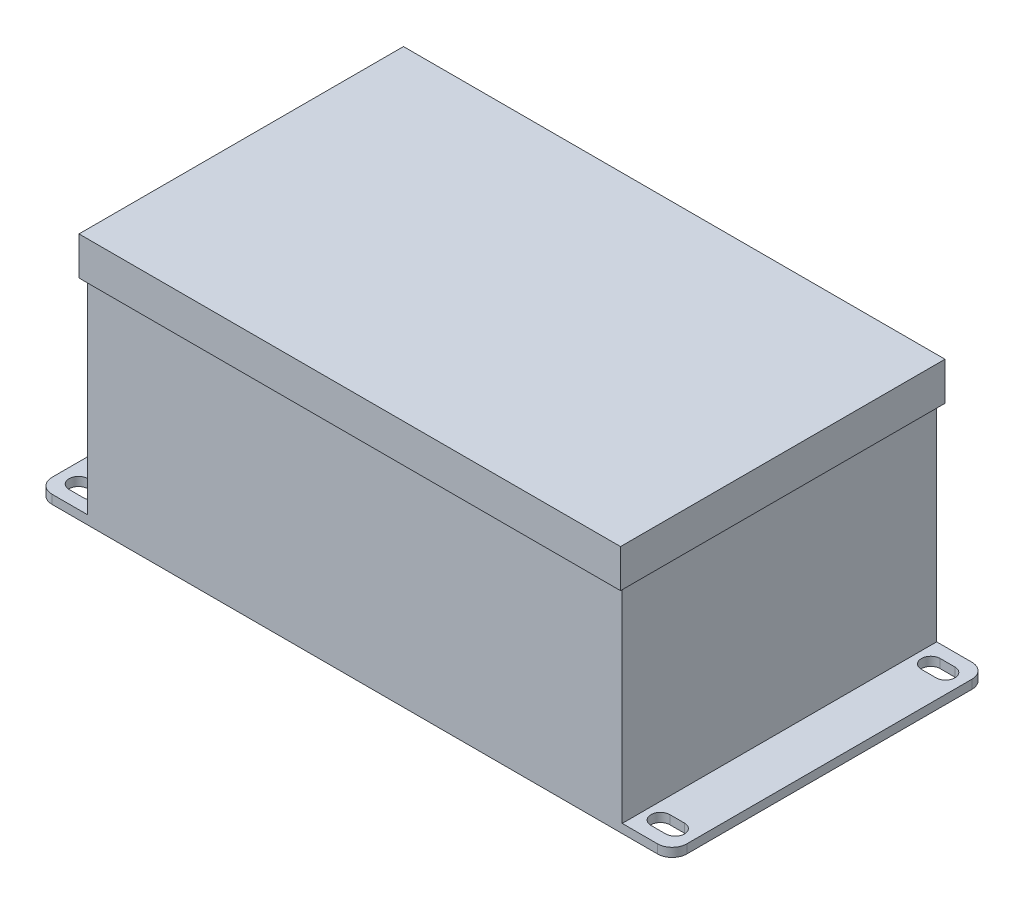
from build123d import *

# Parameters (mm, degrees)
BOSS_EXTRUDE1_DEPTH = 3
SKETCH2_W           = 182
SKETCH2_H           = 107
BOSS_EXTRUDE2_DEPTH = 70
SKETCH4_W           = 184.261814912
SKETCH4_H           = 110.411316032
BOSS_EXTRUDE3_DEPTH = 13


with BuildPart() as part:
    # Sketch1 → Boss-Extrude1 (new body)
    with BuildSketch(Plane(origin=(0, 0, 0), x_dir=(1, 0, 0), z_dir=(0, 1, 0))):
        with BuildLine():
            Line((-103, -53.5), (103, -53.5))
            ThreePointArc((103, -53.5), (106.535533906, -52.035533906), (108, -48.5))
            Line((108, -48.5), (108, 48.5))
            ThreePointArc((108, 48.5), (106.535533906, 52.035533906), (103, 53.5))
            Line((103, 53.5), (-103, 53.5))
            ThreePointArc((-103, 53.5), (-106.535533906, 52.035533906), (-108, 48.5))
            Line((-108, 48.5), (-108, -48.5))
            ThreePointArc((-108, -48.5), (-106.535533906, -52.035533906), (-103, -53.5))
        make_face()
        with BuildLine():
            Line((-101.5, 49.2), (-96.5, 49.2))
            ThreePointArc((-96.5, 49.2), (-93.3, 46), (-96.5, 42.8))
            Line((-96.5, 42.8), (-101.5, 42.8))
            ThreePointArc((-101.5, 42.8), (-104.7, 46), (-101.5, 49.2))
        make_face(mode=Mode.SUBTRACT)
        with BuildLine():
            Line((96.5, 49.2), (101.5, 49.2))
            ThreePointArc((101.5, 49.2), (104.7, 46), (101.5, 42.8))
            Line((101.5, 42.8), (96.5, 42.8))
            ThreePointArc((96.5, 42.8), (93.3, 46), (96.5, 49.2))
        make_face(mode=Mode.SUBTRACT)
        with BuildLine():
            Line((-101.5, -42.8), (-96.5, -42.8))
            ThreePointArc((-96.5, -42.8), (-93.3, -46), (-96.5, -49.2))
            Line((-96.5, -49.2), (-101.5, -49.2))
            ThreePointArc((-101.5, -49.2), (-104.7, -46), (-101.5, -42.8))
        make_face(mode=Mode.SUBTRACT)
        with BuildLine():
            Line((96.5, -42.8), (101.5, -42.8))
            ThreePointArc((101.5, -42.8), (104.7, -46), (101.5, -49.2))
            Line((101.5, -49.2), (96.5, -49.2))
            ThreePointArc((96.5, -49.2), (93.3, -46), (96.5, -42.8))
        make_face(mode=Mode.SUBTRACT)
    extrude(amount=BOSS_EXTRUDE1_DEPTH)

    # Sketch2 → Boss-Extrude2 (add)
    with BuildSketch(Plane(origin=(0, 3, 0), x_dir=(1, 0, 0), z_dir=(0, 1, 0))):
        Rectangle(SKETCH2_W, SKETCH2_H)
    extrude(amount=BOSS_EXTRUDE2_DEPTH)

    # Sketch4 → Boss-Extrude3 (add)
    with BuildSketch(Plane(origin=(0, 73, 0), x_dir=(1, 0, 0), z_dir=(0, 1, 0))):
        Rectangle(SKETCH4_W, SKETCH4_H)
    extrude(amount=BOSS_EXTRUDE3_DEPTH)


solid = part.part
